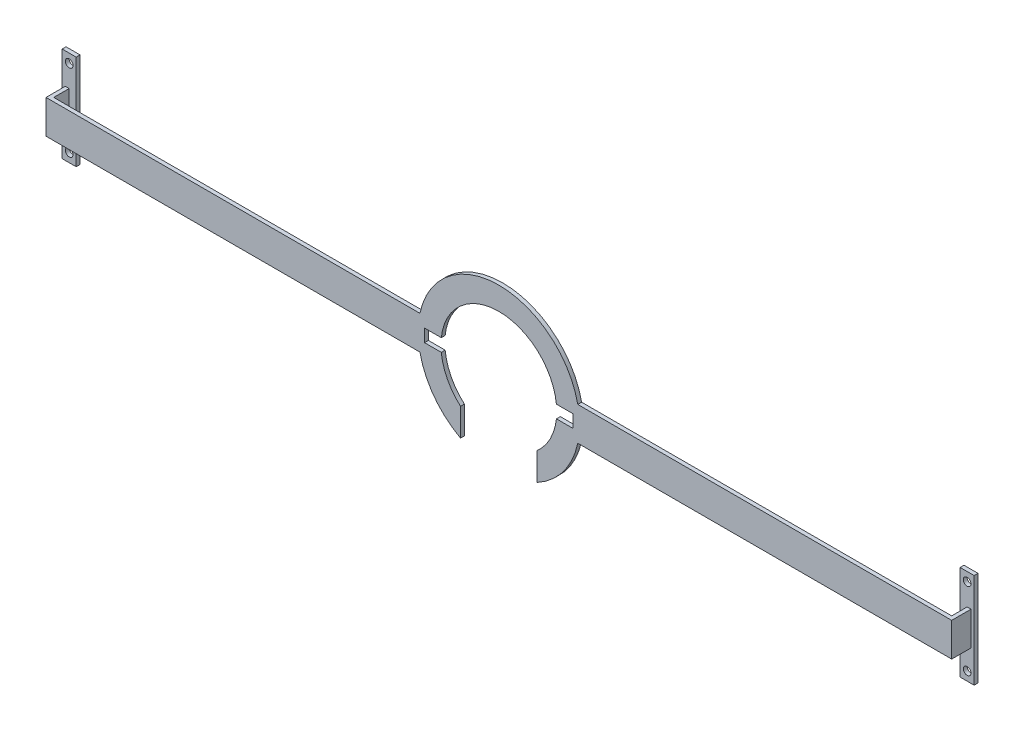
SolidWorks part; units mm, degrees
ref_plane "Front Plane" through (0, 0, 0) normal (0, 0, 1) x (1, 0, 0)
ref_plane "Top Plane" through (0, 0, 0) normal (0, 1, 0) x (1, 0, 0)
ref_plane "Right Plane" through (0, 0, 0) normal (1, 0, 0) x (0, 0, -1)
sketch "Sketch1" plane through (0, 0, 0) normal (0, 0, 1) x (1, 0, 0)
  line L0 (20.4452, 4.3489) -> (117.2753, 4.3489)
  line L1 (-117.2753, 4.3489) -> (-20.4452, 4.3489)
  line L2 (-117.2753, 4.3489) -> (-117.2753, -4.3489)
  line L3 (-117.2753, -4.3489) -> (-20.4452, -4.3489)
  line L4 (117.2753, 4.3489) -> (117.2753, -4.3489)
  line L5 (-117.2753, 4.3489) -> (117.2753, -4.3489) construction
  line L6 (-117.2753, -4.3489) -> (117.2753, 4.3489) construction
  line L7 (-19.2443, -1.6414) -> (-14.9099, -1.6414)
  line L8 (-19.2443, -1.6414) -> (-19.2443, 1.6414)
  line L9 (-19.2443, 1.6414) -> (-14.9099, 1.6414)
  line L10 (19.2443, -1.6414) -> (19.2443, 1.6414)
  line L11 (-19.2443, -1.6414) -> (19.2443, 1.6414) construction
  line L12 (-19.2443, 1.6414) -> (19.2443, -1.6414) construction
  line L13 (20.4452, -4.3489) -> (117.2753, -4.3489)
  line L14 (14.9099, 1.6414) -> (19.2443, 1.6414)
  line L15 (14.9099, -1.6414) -> (19.2443, -1.6414)
  line L18 (-9.9274, -11.2448) -> (-9.9274, -18.3947)
  line L20 (9.9274, -11.2448) -> (9.9274, -18.3947)
  line L21 (-9.9274, -6.7842) -> (9.9274, -23.2158) construction
  line L22 (0, -15) -> (9.9274, -6.7842) construction
  arc A0 (9.9274, -11.2448) -> (14.9099, -1.6414) centre (0, 0) ccw
  arc A1 (-20.4452, -4.3489) -> (-9.9274, -18.3947) centre (0, 0) ccw
  arc A2 (20.4452, 4.3489) -> (-20.4452, 4.3489) centre (0, 0) ccw
  arc A3 (-14.9099, -1.6414) -> (-9.9274, -11.2448) centre (0, 0) ccw
  arc A4 (14.9099, 1.6414) -> (-14.9099, 1.6414) centre (0, 0) ccw
  arc A5 (9.9274, -18.3947) -> (20.4452, -4.3489) centre (0, 0) ccw
  point P0 (0, 0)
  point P7 (0, -15)
extrude "Boss-Extrude1" add sketch "Sketch1" against normal blind 1 contours A2 L1 L2 L3 A1 L13 L4 L0
sketch "Sketch2" plane through (0, 0, 0) normal (0, 0, 1) x (1, 0, 0)
  line L0 (-117.2753, -4.3489) -> (-20.4452, -4.3489) construction
  line L1 (-117.2753, 4.3489) -> (-116.2753, 4.3489)
  line L2 (-117.2753, 4.3489) -> (-117.2753, -4.3489)
  line L3 (-117.2753, -4.3489) -> (-116.2753, -4.3489)
  line L4 (-116.2753, 4.3489) -> (-116.2753, -4.3489)
  line L5 (20.4452, -4.3489) -> (117.2753, -4.3489) construction
  line L6 (117.2753, 4.3489) -> (116.2753, 4.3489)
  line L7 (117.2753, 4.3489) -> (117.2753, -4.3489)
  line L8 (117.2753, -4.3489) -> (116.2753, -4.3489)
  line L9 (116.2753, 4.3489) -> (116.2753, -4.3489)
extrude "Boss-Extrude2" add sketch "Sketch2" against normal up to surface (6 mm away)
sketch "Sketch3" plane through (0, 0, -6) normal (0, 0, 1) x (1, 0, 0)
  line L0 (-116.2753, 4.3489) -> (-116.2753, -4.3489) construction
  line L1 (-118.0882, 12.2989) -> (-114.4624, 12.2989)
  line L2 (-118.0882, 12.2989) -> (-118.0882, -12.2989)
  line L3 (-118.0882, -12.2989) -> (-114.4624, -12.2989)
  line L4 (-114.4624, 12.2989) -> (-114.4624, -12.2989)
  line L5 (-118.0882, 12.2989) -> (-114.4624, -12.2989) construction
  line L6 (-118.0882, -12.2989) -> (-114.4624, 12.2989) construction
  line L7 (0, 0) -> (0, -37.7226) construction
  line L8 (118.0882, -12.2989) -> (114.4624, 12.2989) construction
  line L9 (118.0882, 12.2989) -> (114.4624, -12.2989) construction
  line L10 (114.4624, 12.2989) -> (114.4624, -12.2989)
  line L11 (118.0882, -12.2989) -> (114.4624, -12.2989)
  line L12 (118.0882, 12.2989) -> (118.0882, -12.2989)
  line L13 (118.0882, 12.2989) -> (114.4624, 12.2989)
  circle A0 centre (-116.2753, -10) radius 1
  circle A1 centre (-116.2753, 10) radius 1
  circle A2 centre (116.2753, 10) radius 1
  circle A3 centre (116.2753, -10) radius 1
  point P0 (-116.2753, 0)
  point P22 (116.2753, 0)
  dimension "D1" = 10
  dimension "D2" = 10
extrude "Boss-Extrude3" add sketch "Sketch3" along normal blind 1 contours L4 L3 L2 L1
